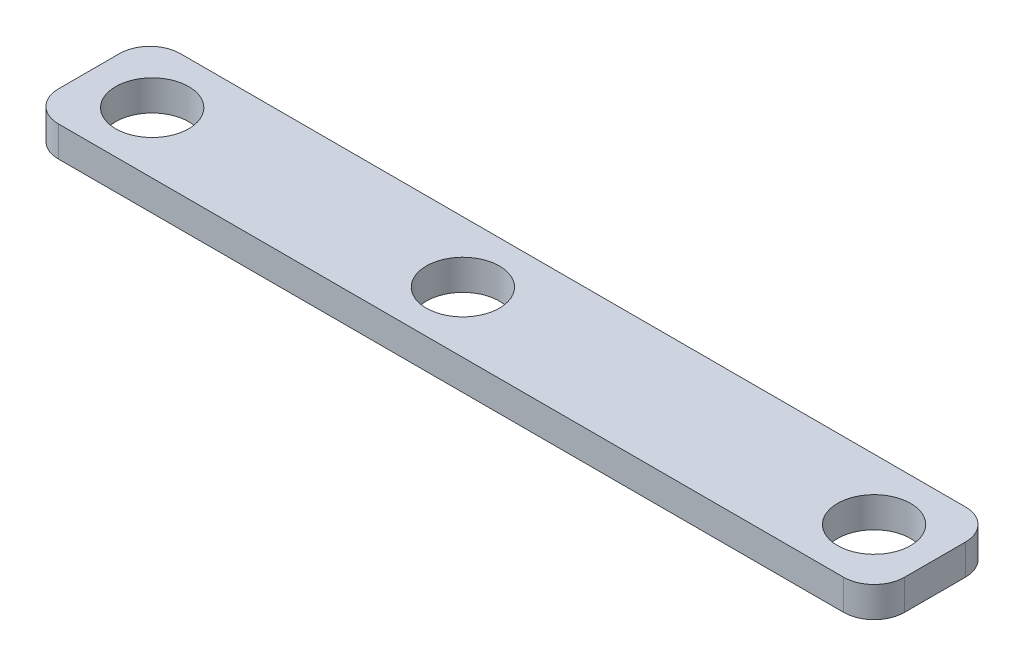
SolidWorks part; units mm, degrees
ref_plane "Front Plane" through (0, 0, 0) normal (0, 0, 1) x (1, 0, 0)
ref_plane "Top Plane" through (0, 0, 0) normal (0, 1, 0) x (1, 0, 0)
ref_plane "Right Plane" through (0, 0, 0) normal (1, 0, 0) x (0, 0, -1)
other "Configuration Table"
sketch "Sketch1" plane through (0, 0, 0) normal (0, 1, 0) x (1, 0, 0)
  line L1 (-150, 20) -> (150, 20)
  line L2 (-150, 20) -> (-150, -20)
  line L3 (-150, -20) -> (150, -20)
  line L4 (150, 20) -> (150, -20)
  line L5 (-150, 20) -> (150, -20) construction
  line L6 (-150, -20) -> (150, 20) construction
  circle A0 centre (130, 0) radius 12
  circle A1 centre (-5, 0) radius 12
  circle A2 centre (-107, 0) radius 12
  point P0 (0, 0)
  dimension "D3" = 24
  dimension "D4" = 20
  dimension "D5" = 24
  dimension "D6" = 135
  dimension "D7" = 24
  dimension "D8" = 102
  dimension "D1" = 300
  dimension "D2" = 40
extrude "Boss-Extrude1" add sketch "Sketch1" along normal blind 10
sketch "Sketch2" plane through (0, 10, 0) normal (0, 1, 0) x (1, 0, 0)
  line L0 (-150, -20) -> (150, -20) construction
  line L1 (-150, 20) -> (-127.7435, 20)
  line L2 (-150, 20) -> (-150, -20)
  line L3 (-150, -20) -> (-127.7435, -20)
  line L4 (-127.7435, 20) -> (-127.7435, -20)
extrude "Cut-Extrude1" cut sketch "Sketch2" against normal blind 10
fillet "Fillet1" radius 10 4 edges at (150, 5, 20) (150, 5, -20) (-127.7435, 5, 20) (-127.7435, 5, -20)
